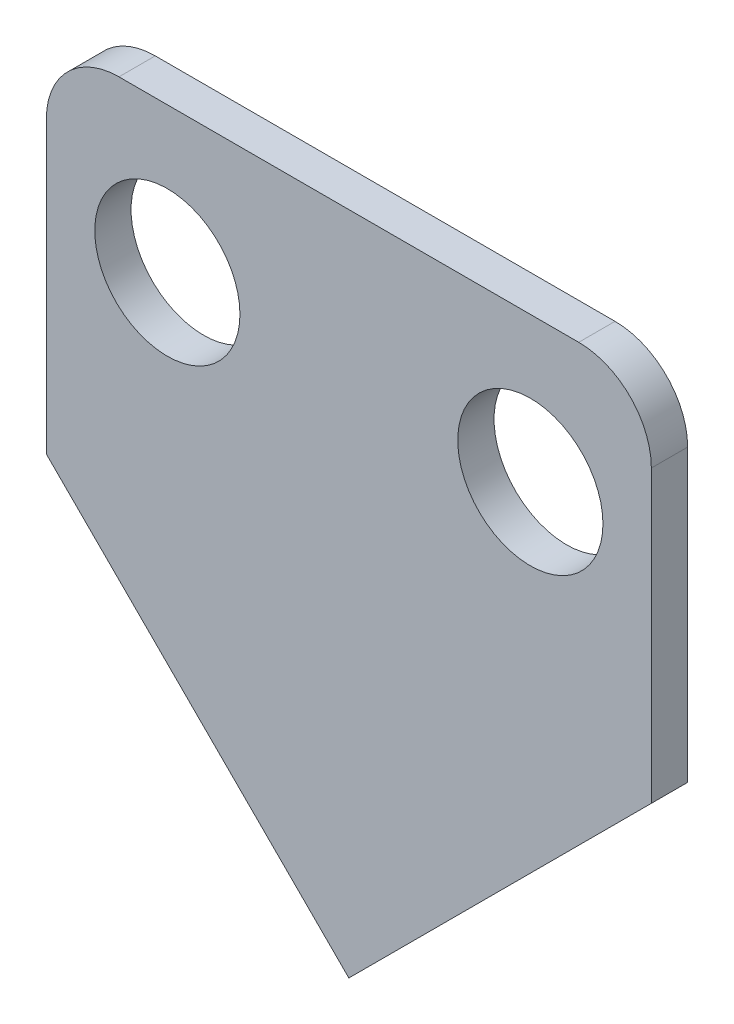
SolidWorks part; units mm, degrees
ref_plane "前视基准面" through (0, 0, 0) normal (0, 0, 1) x (1, 0, 0)
ref_plane "上视基准面" through (0, 0, 0) normal (0, 1, 0) x (1, 0, 0)
ref_plane "右视基准面" through (0, 0, 0) normal (1, 0, 0) x (0, 0, -1)
sketch "草图1" plane through (0, 0, 0) normal (0, 0, 1) x (1, 0, 0)
  line L0 (-12.5, 0) -> (12.5, 0)
  line L1 (12.5, 0) -> (12.5, -15)
  line L2 (-12.5, -15) -> (0, -27.5)
  line L3 (0, -27.5) -> (12.5, -15)
  line L6 (-12.5, -15) -> (-12.5, 0)
  line L7 (0, 0) -> (0, -88.4502) construction
  dimension "D1" = 25
  dimension "D2" = 15
  dimension "D3" = 135
extrude "凸台-拉伸1" add sketch "草图1" along normal blind 1.5
hole_wizard "Ø6.0 (6) 直径孔1" positions "草图3" profile "草图2" hole size "Ø6.0" standard "GB" end condition through all
sketch "草图3" plane through (0, 0, 1.5) normal (0, 0, 1) x (1, 0, 0)
  line L0 (0, 0) -> (0, -28.6169) construction
  line L2 (12.5, 0) -> (-12.5, 0) construction
  point P0 (-7.5, -6)
  point P2 (7.5, -6)
  dimension "D1" = 15
  dimension "D2" = 6
sketch "草图2" plane through (-7.5, -6, 1.5) normal (1, 0, 0) x (0, -1, 0)
  line L0 (0, 0) -> (0, 1.5)
  line L1 (0, 1.5) -> (3, 1.5)
  line L2 (3, 1.5) -> (3, 0)
  line L5 (3, 0) -> (0, 0)
  line L11 (0, -6.35) -> (0, 107.95) construction
  dimension "通孔孔直径" = 6
  dimension "通孔孔深度" = 1.5
fillet "圆角1" radius 3 2 edges at (12.5, 0, 0.75) (-12.5, 0, 0.75)
